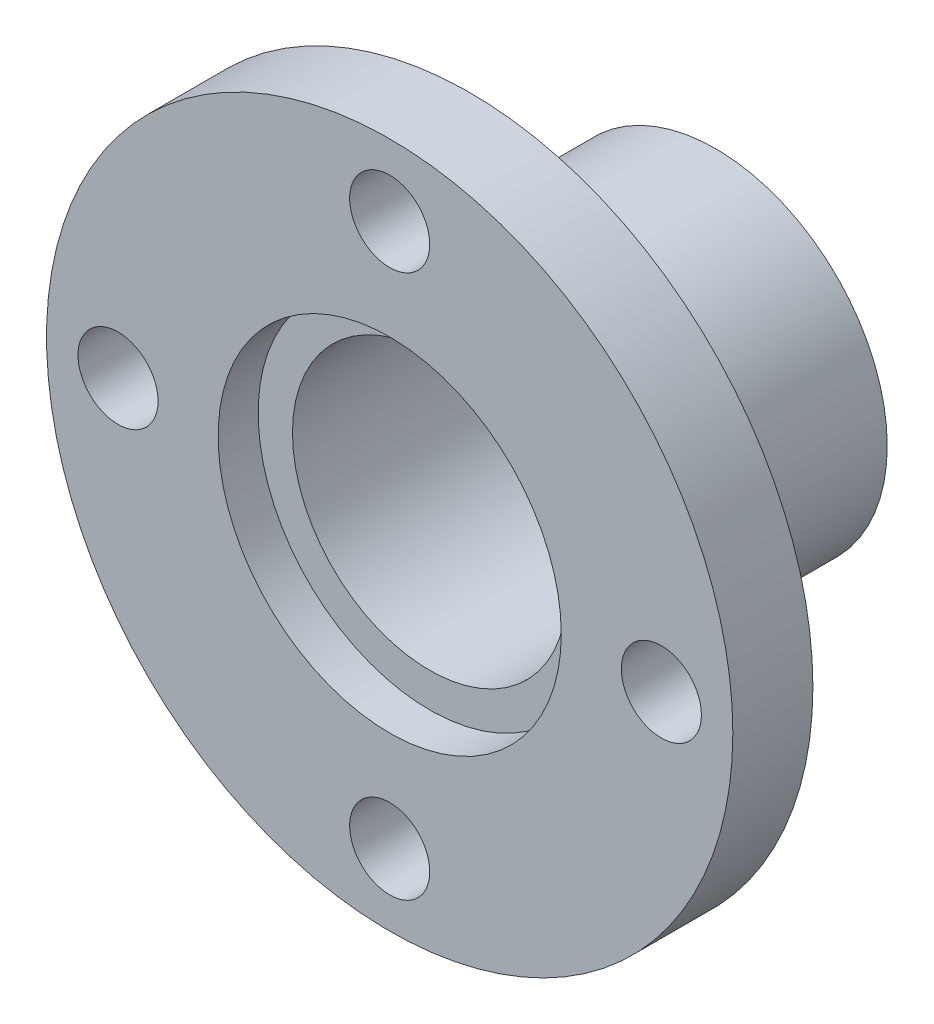
from build123d import *

# Parameters (mm, degrees)
SKETCH1_R                           = 30
SKETCH1_R_2                         = 24
EXTRUDE_THIN1_DEPTH                 = 50
SKETCH2_R                           = 60
SKETCH2_R_2                         = 30
BOSS_EXTRUDE1_DEPTH                 = 7
SKETCH4_W                           = 7
SKETCH4_H                           = 14.001
F_14_0_14_DIAMETER_HOLE1_AT_2_COUNT = 2
F_14_0_14_DIAMETER_HOLE1_AT_2_PITCH = 67.175144213
F_14_0_14_DIAMETER_HOLE1_AT_3_COUNT = 2
F_14_0_14_DIAMETER_HOLE1_AT_3_PITCH = 67.175144213
F_14_0_14_DIAMETER_HOLE1_AT_4_COUNT = 2
F_14_0_14_DIAMETER_HOLE1_AT_4_PITCH = 95


with BuildPart() as part:
    # Sketch1 → Extrude-Thin1 (new body)
    with BuildSketch(Plane.XY):
        Circle(SKETCH1_R)
        Circle(SKETCH1_R_2, mode=Mode.SUBTRACT)
    extrude(amount=EXTRUDE_THIN1_DEPTH)


with BuildPart() as body_2:
    # Sketch2 → Boss-Extrude1 (new, symmetric)
    with BuildSketch(Plane.XY.offset(50)):
        Circle(SKETCH2_R)
        Circle(SKETCH2_R_2, mode=Mode.SUBTRACT)
    extrude(amount=BOSS_EXTRUDE1_DEPTH, both=True)

    # Sketch4 → Ø14.0 (14) Diameter Hole1 (revolve, cut)
    with BuildSketch(Plane(origin=(0, 47.5, 57), x_dir=(0, -1, 0), z_dir=(1, 0, 0))):
        with Locations((3.5, 7.0005)):
            Rectangle(SKETCH4_W, SKETCH4_H)
    f_14_0_14_diameter_hole1 = revolve(axis=Axis((0, 47.5, 63.35), (0, 0, -1)), mode=Mode.SUBTRACT)

    # Ø14.0 (14) Diameter Hole1 at 2: Ø14.0 (14) Diameter Hole1 ×2
    with Locations(*[Vector(-0.7071067811865476, -0.7071067811865476, 0) * (i * F_14_0_14_DIAMETER_HOLE1_AT_2_PITCH) for i in range(1, F_14_0_14_DIAMETER_HOLE1_AT_2_COUNT)]):
        add(f_14_0_14_diameter_hole1, mode=Mode.SUBTRACT)

    # Ø14.0 (14) Diameter Hole1 at 3: Ø14.0 (14) Diameter Hole1 ×2
    with Locations(*[Vector(0.7071067811865476, -0.7071067811865476, 0) * (i * F_14_0_14_DIAMETER_HOLE1_AT_3_PITCH) for i in range(1, F_14_0_14_DIAMETER_HOLE1_AT_3_COUNT)]):
        add(f_14_0_14_diameter_hole1, mode=Mode.SUBTRACT)

    # Ø14.0 (14) Diameter Hole1 at 4: Ø14.0 (14) Diameter Hole1 ×2
    with Locations(*[(0, -i * F_14_0_14_DIAMETER_HOLE1_AT_4_PITCH, 0) for i in range(1, F_14_0_14_DIAMETER_HOLE1_AT_4_COUNT)]):
        add(f_14_0_14_diameter_hole1, mode=Mode.SUBTRACT)


solid = Compound([part.part, body_2.part])
